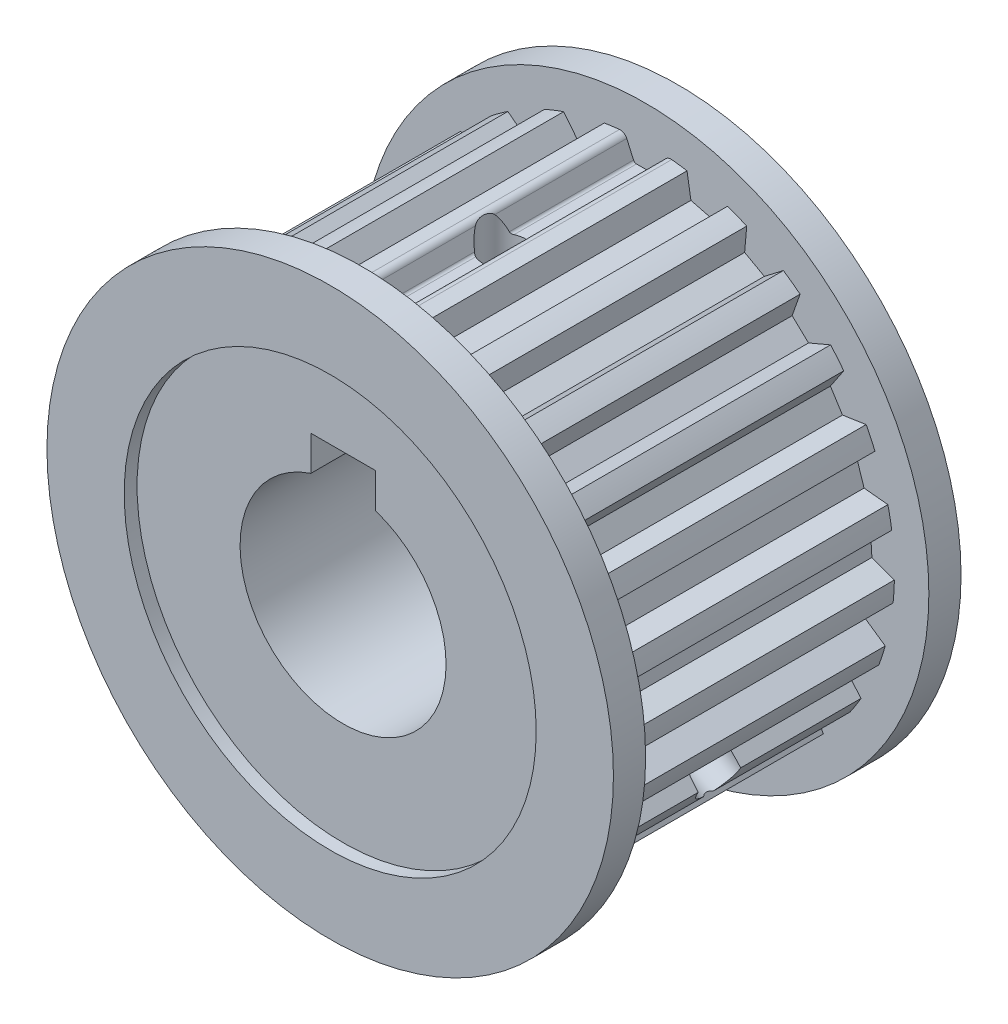
SolidWorks part; units mm, degrees
ref_plane "前视基准面" through (0, 0, 0) normal (0, 0, 1) x (1, 0, 0)
ref_plane "上视基准面" through (0, 0, 0) normal (0, 1, 0) x (1, 0, 0)
ref_plane "右视基准面" through (0, 0, 0) normal (1, 0, 0) x (0, 0, -1)
sketch "草图1" plane through (0, 0, 0) normal (0, 0, 1) x (1, 0, 0)
  circle A0 centre (0, 0) radius 19.325
  dimension "D1" = 38.65
extrude "凸台-拉伸1" add sketch "草图1" along normal mid plane 27
sketch "草图2" plane through (0, 0, 0) normal (0, 0, 1) x (1, 0, 0)
  line L0 (-0.875, 17.555) -> (0.875, 17.555)
  line L1 (-0.875, 17.555) -> (-1.625, 19.2566)
  line L2 (0.875, 17.555) -> (1.625, 19.2566)
  arc A0 (1.625, 19.2566) -> (-1.625, 19.2566) centre (0, 0) ccw
  circle A2 centre (0, 0) radius 19.325 construction
  dimension "D1" = 0.875
  dimension "D2" = 0.875
  dimension "D3" = 1.75
  dimension "D4" = 3.25
  dimension "D5" = 1.625
  dimension "D6" = 17.555
extrude "切除-拉伸1" cut sketch "草图2" against normal mid plane 27
fillet "圆角3" radius 0.55 2 edges at (1.625, 19.2566, 0) (-1.625, 19.2566, 0)
fillet "圆角4" radius 0.25 2 edges at (-0.875, 17.555, 0) (0.875, 17.555, 0)
pattern_circular "阵列(圆周)2" count 25 over 360 about axis through (0, 0, 0) along (0, 0, 1) of "切除-拉伸1"
sketch "草图3" plane through (0, 0, 13.5) normal (0, 0, 1) x (1, 0, 0)
  circle A0 centre (0, 0) radius 22
  dimension "D1" = 44
extrude "凸台-拉伸2" add sketch "草图3" against normal blind 2.5
mirror "镜向1" about plane through (0, 0, 0) normal (0, 0, 1) of "凸台-拉伸2"
sketch "草图4" plane through (0, 0, 13.5) normal (0, 0, 1) x (1, 0, 0)
  circle A0 centre (0, 0) radius 16
  dimension "D1" = 32
extrude "切除-拉伸2" cut sketch "草图4" against normal blind 1
mirror "镜向2" about plane through (0, 0, 0) normal (0, 0, 1) of "切除-拉伸2"
sketch "草图5" plane through (0, 0, 0) normal (0, 0, 1) x (1, 0, 0)
  line L1 (-2.5, 10.3) -> (2.5, 10.3)
  line L2 (-2.5, 10.3) -> (-2.5, 7.5993)
  line L4 (2.5, 10.3) -> (2.5, 7.5993)
  arc A0 (-2.5, 7.5993) -> (2.5, 7.5993) centre (0, 0) ccw
  dimension "D1" = 16
  dimension "D4" = 10.3
  dimension "D2" = 5
  dimension "D3" = 2.5
extrude "切除-拉伸3" cut sketch "草图5" against normal mid plane 27 contours L2 A0 L4 L1
hole_wizard "M4 螺纹孔1" positions "草图7" profile "草图6" tap size "M4" standard "ISO"
sketch "草图7" plane through (0, 0, 0) normal (0, -1, 0) x (-1, 0, 0)
  point P0 (0, 0)
sketch "草图6" plane through (0, 0, 0) normal (1, 0, 0) x (0, 0, -1)
  line L0 (0, 0) -> (0, 30.0526)
  line L1 (0, 30.0526) -> (1.65, 30.0526)
  line L2 (1.65, 30.0526) -> (1.65, 0)
  line L5 (1.65, 0) -> (0, 0)
  line L11 (0, -6.35) -> (0, 107.95) construction
  dimension "通孔螺纹孔钻头直径" = 3.3
  dimension "通孔螺纹孔钻头深度" = 30.0526
cosmetic thread "孔螺蚊线1" parameters "D2"=4
pattern_circular "阵列(圆周)3" count 2 every 120 about axis through (0, 0, 13.5) along (0, 0, -1) of "M4 螺纹孔1"
